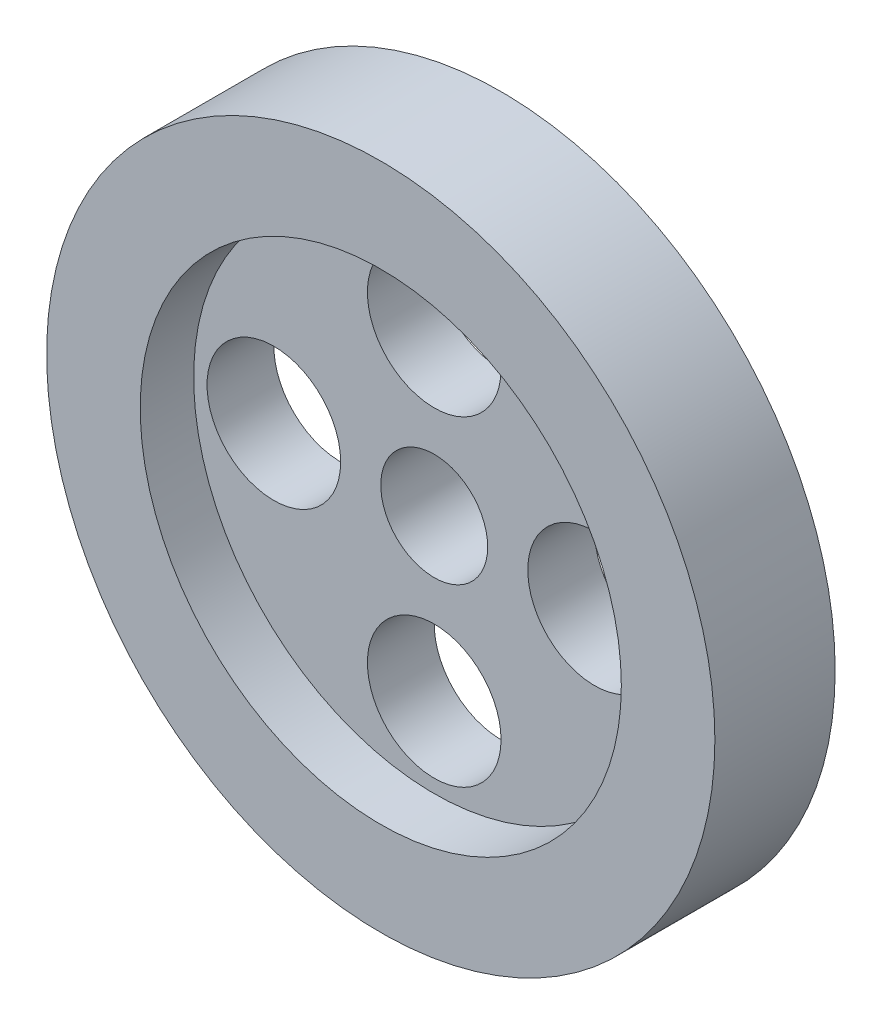
SolidWorks part; units mm, degrees
ref_plane "Front Plane" through (0, 0, 0) normal (0, 0, 1) x (1, 0, 0)
ref_plane "Top Plane" through (0, 0, 0) normal (0, 1, 0) x (1, 0, 0)
ref_plane "Right Plane" through (0, 0, 0) normal (1, 0, 0) x (0, 0, -1)
other "Configuration Table"
sketch "Sketch1" plane through (0, 0, 0) normal (0, 0, 1) x (1, 0, 0)
  circle A0 centre (0, 0) radius 25
  dimension "D1" = 50
extrude "Boss-Extrude1" add sketch "Sketch1" along normal blind 9
sketch "Sketch2" plane through (0, 0, 9) normal (0, 0, 1) x (1, 0, 0)
  circle A0 centre (0, 0) radius 18
  dimension "D1" = 36
extrude "Cut-Extrude1" cut sketch "Sketch2" against normal blind 4
sketch "Sketch3" plane through (0, 0, 5) normal (0, 0, 1) x (1, 0, 0)
  circle A0 centre (0, 0) radius 12 construction
  circle A1 centre (0, 12) radius 5
  circle A2 centre (12, 0) radius 5
  circle A3 centre (0, -12) radius 5
  circle A4 centre (-12, 0) radius 5
  point P14 (0, 0)
  dimension "D1" = 24
  dimension "D2" = 10
  dimension "D3" = 4
extrude "Cut-Extrude2" cut sketch "Sketch3" against normal through all
sketch "Sketch4" plane through (0, 0, 5) normal (0, 0, 1) x (1, 0, 0)
  circle A0 centre (0, 0) radius 4
  dimension "D1" = 8
extrude "Cut-Extrude3" cut sketch "Sketch4" against normal through all
sketch "Sketch5" plane through (0, 0, 0) normal (0, 0, -1) x (-1, 0, 0)
  circle A0 centre (0, 0) radius 6
  circle A1 centre (0, 0) radius 4
  dimension "D1" = 12
extrude "Boss-Extrude2" add sketch "Sketch5" along normal blind 1
